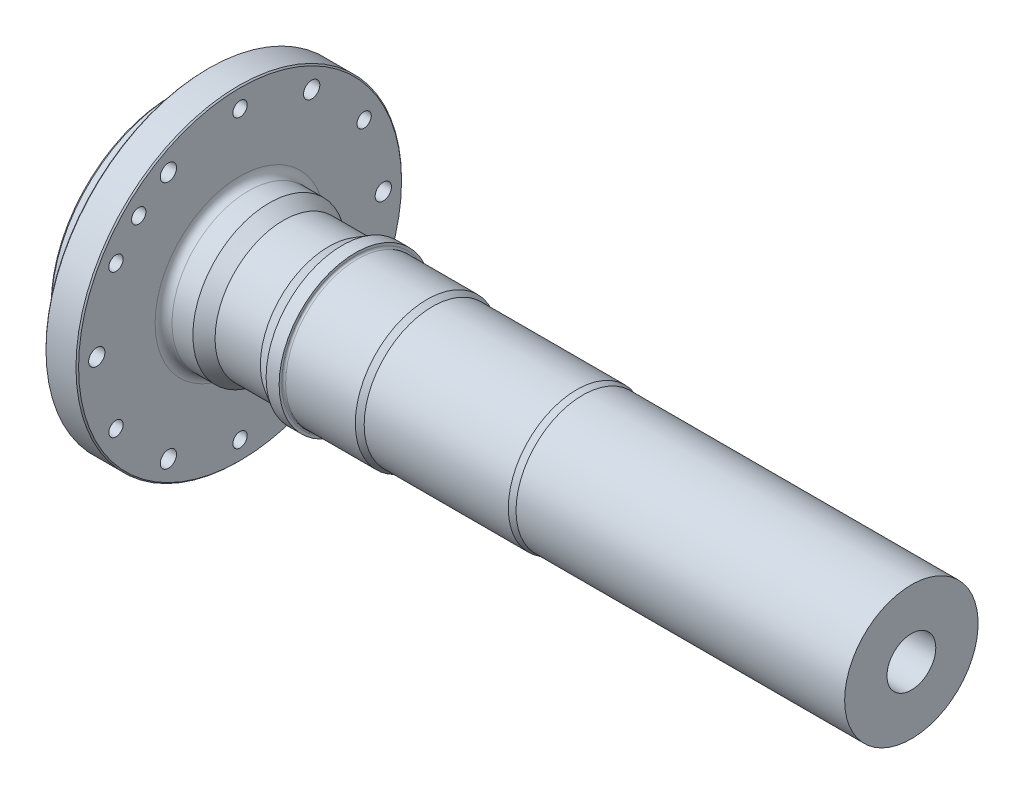
SolidWorks part; units mm, degrees
material "1.6571 (20NiCrMoS6-4)"
ref_plane "Front Plane" through (0, 0, 0) normal (0, 0, 1) x (1, 0, 0)
ref_plane "Top Plane" through (0, 0, 0) normal (0, 1, 0) x (1, 0, 0)
ref_plane "Right Plane" through (0, 0, 0) normal (1, 0, 0) x (0, 0, -1)
sketch "Sketch1" plane through (0, 0, 0) normal (0, 0, 1) x (1, 0, 0)
  line L0 (0, 0) -> (1156.519, 0) construction
  line L1 (0, 0) -> (0, 185)
  line L2 (5, 190) -> (47, 190)
  line L3 (55, 198) -> (55, 248)
  line L4 (57, 250) -> (103, 250)
  line L5 (105, 248) -> (105, 130.475)
  line L6 (118, 117.475) -> (150, 117.475)
  line L7 (150, 117.475) -> (171.6073, 105)
  line L8 (171.6073, 105) -> (241.2154, 105)
  line L9 (241.2154, 105) -> (262, 117)
  line L10 (262, 117) -> (282, 117)
  line L11 (282, 117) -> (282, 113)
  line L12 (285, 110) -> (392, 110)
  line L13 (392, 110) -> (400.6603, 105)
  line L14 (400.6603, 105) -> (622, 105)
  line L15 (622, 105) -> (631.3301, 102.5)
  line L16 (631.3301, 102.5) -> (1136, 102.5)
  line L17 (1136, 102.5) -> (1136, 0)
  line L18 (55, 248) -> (57, 250)
  line L19 (103, 250) -> (105, 248)
  line L20 (0, 185) -> (5, 190)
  line L21 (47.8, 189.2) -> (53.8, 189.2)
  line L22 (55.8, 191.2) -> (55.8, 197.2)
  line L23 (55.8, 197.2) -> (55, 198)
  line L24 (47.8, 189.2) -> (47, 190)
  line L25 (0, 0) -> (1136, 0)
  arc A0 (105, 130.475) -> (118, 117.475) centre (118, 130.475) ccw
  arc A1 (53.8, 189.2) -> (55.8, 191.2) centre (53.8, 191.2) ccw
  arc A2 (282, 113) -> (285, 110) centre (285, 113) ccw
  point P3 (26, 190)
  point P4 (0, 190)
  point P6 (55, 250)
  point P7 (105, 250)
  dimension "D21" = 13
  dimension "D31" = 2
  dimension "D32" = 3
  dimension "D1" = 55
  dimension "D2" = 50
  dimension "D3" = 190
  dimension "D4" = 117.475
  dimension "D5" = 250
  dimension "D6" = 30
  dimension "D7" = 105
  dimension "D8" = 45
  dimension "D9" = 177
  dimension "D10" = 20
  dimension "D11" = 30
  dimension "D12" = 117
  dimension "D13" = 110
  dimension "D14" = 110
  dimension "D15" = 30
  dimension "D16" = 105
  dimension "D17" = 230
  dimension "D18" = 15
  dimension "D19" = 514
  dimension "D20" = 102.5
  dimension "D22" = 0.8
  dimension "D23" = 45
  dimension "D27" = 0.8
  dimension "D28" = 45
  dimension "D29" = 8
  dimension "D30" = 8
revolve "Revolve1" add sketch "Sketch1" angle 360 about L0
sketch "Sketch2" plane through (55, 0, 0) normal (-1, 0, 0) x (0, 0, 1)
  line L0 (0, 0) -> (0, 220) construction
  line L1 (0, 0) -> (190.5256, 110) construction
  line L2 (0, 0) -> (190.5256, -110) construction
  line L3 (0, 0) -> (0, -220) construction
  line L4 (0, 0) -> (-190.5256, -110) construction
  line L5 (0, 0) -> (-190.5256, 110) construction
  line L6 (0, 0) -> (155.5635, 155.5635) construction
  line L7 (0, 0) -> (-155.5635, -155.5635) construction
  line L8 (0, 0) -> (-110, 190.5256) construction
  circle A0 centre (0, 0) radius 220 construction
  circle A1 centre (-110, 190.5256) radius 12.5
  circle A2 centre (110, 190.5256) radius 12.5
  circle A3 centre (220, 0) radius 12.5
  circle A4 centre (110, -190.5256) radius 12.5
  circle A5 centre (-110, -190.5256) radius 12.5
  circle A6 centre (-220, 0) radius 12.5
  point P11 (0, 0)
  point P27 (0, 0)
  dimension "D1" = 440
  dimension "D5" = 25
  dimension "D3" = 45
  dimension "D4" = 30
  dimension "D2" = 6
  dimension "D6" = 6
hole_wizard "M24x2.0 Tapped Hole1" positions "3DSketch1" profile "Sketch3" tap size "M24x2.0" standard "GB" end condition through all
sketch3d "3DSketch1"
  point P0 (55, 220, 0)
  point P3 (55, 110, 190.5256)
  point P6 (55, 110, -190.5256)
  point P9 (55, -110, -190.5256)
  point P12 (55, -220, 0)
  point P15 (55, -110, 190.5256)
  point P19 (55, 155.5635, 155.5635)
  point P22 (55, -155.5635, -155.5635)
sketch "Sketch3" plane through (55, 220, 0) normal (0, 1, 0) x (0, 0, 1)
  line L0 (0, 0) -> (0, 1081)
  line L1 (0, 1081) -> (11, 1081)
  line L2 (11, 1081) -> (11, 0)
  line L5 (11, 0) -> (0, 0)
  line L11 (0, -6.35) -> (0, 107.95) construction
  dimension "通孔螺纹孔钻头直径" = 22
  dimension "通孔螺纹孔钻头深度" = 1081
cosmetic thread "CosmeticThread hole thread 1" parameters "D2"=24
cosmetic thread "CosmeticThread hole thread 2" parameters "D2"=24
cosmetic thread "CosmeticThread hole thread 3" parameters "D2"=24
cosmetic thread "CosmeticThread hole thread 4" parameters "D2"=24
cosmetic thread "CosmeticThread hole thread 5" parameters "D2"=24
cosmetic thread "CosmeticThread hole thread 6" parameters "D2"=24
cosmetic thread "CosmeticThread hole thread 7" parameters "D2"=24
cosmetic thread "CosmeticThread hole thread 8" parameters "D2"=24
extrude "Cut-Extrude1" cut sketch "Sketch2" against normal through all
sketch "Sketch4" plane through (1136, 0, 0) normal (1, 0, 0) x (0, 0, -1)
  circle A0 centre (0, 0) radius 37.5
  dimension "D1" = 75
extrude "Cut-Extrude2" cut sketch "Sketch4" against normal through all
sketch "Sketch5" plane through (0, 0, 0) normal (1, 0, 0) x (0, 0, -1)
  line L0 (0, 0) -> (0, 266.3965) construction
